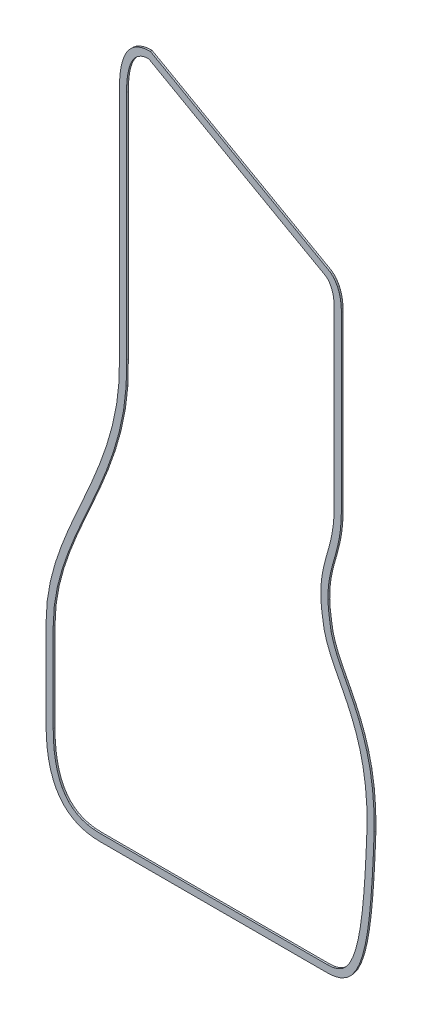
from build123d import *

# Parameters (mm, degrees)
EXTRUDE_1_DEPTH = 1.5


with BuildPart() as part:
    # 草图1 → 凸台-拉伸1 (new, symmetric)
    with BuildSketch(Plane.XY):
        Polygon((103, 235), (-24.833333333, 235), (-152.666666667, 235), (-280.5, 235), (-293.035714286, 235.637755102), (-304.642857143, 237.551020408), (-315.321428571, 240.739795918), (-325.071428571, 245.204081633), (-333.892857143, 250.943877551), (-341.785714286, 257.959183673), (-348.75, 266.25), (-354.785714286, 275.816326531), (-359.892857143, 286.658163265), (-364.071428571, 298.775510204), (-367.321428571, 312.168367347), (-369.642857143, 326.836734694), (-371.035714286, 342.780612245), (-371.5, 360), (-371.5, 410), (-371.5, 460), (-371.5, 510), (-369.607325073, 541.716472303), (-364.317784257, 572.711370262), (-356.214103499, 603.18148688), (-345.879008746, 633.32361516), (-333.895225948, 663.334548105), (-320.84548105, 693.411078717), (-307.3125, 723.75), (-293.879008746, 754.548104956), (-281.127733236, 786.002186589), (-269.641399417, 818.309037901), (-260.002733236, 851.665451895), (-252.794460641, 886.268221574), (-248.59930758, 922.314139942), (-248, 960), (-248, 1090), (-248, 1220), (-248, 1350), (-247.734693878, 1361.020408163), (-246.93877551, 1371.224489796), (-245.612244898, 1380.612244898), (-243.755102041, 1389.183673469), (-241.367346939, 1396.93877551), (-238.448979592, 1403.87755102), (-235, 1410), (-231.020408163, 1415.306122449), (-226.510204082, 1419.795918367), (-221.469387755, 1423.469387755), (-215.897959184, 1426.326530612), (-209.795918367, 1428.367346939), (-203.163265306, 1429.591836735), (-196, 1430), (-95.25, 1373.333333333), (5.5, 1316.666666667), (106.25, 1260), (108.93622449, 1257.887755102), (111.423469388, 1255.551020408), (113.711734694, 1252.989795918), (115.801020408, 1250.204081633), (117.691326531, 1247.193877551), (119.382653061, 1243.959183673), (120.875, 1240.5), (122.168367347, 1236.816326531), (123.262755102, 1232.908163265), (124.158163265, 1228.775510204), (124.854591837, 1224.418367347), (125.352040816, 1219.836734694), (125.650510204, 1215.030612245), (125.75, 1210), (125.75, 1113.333333333), (125.75, 1016.666666667), (125.75, 920), (125.280976676, 904.7303207), (123.987609329, 890.903790087), (122.040451895, 878.279883382), (119.610058309, 866.618075802), (116.866982507, 855.677842566), (113.981778426, 845.218658892), (111.125, 835), (108.467201166, 824.781341108), (106.17893586, 814.322157434), (104.430758017, 803.381924198), (103.393221574, 791.720116618), (103.236880466, 779.096209913), (104.13228863, 765.2696793), (106.25, 750), (108.586825802, 735.40451895), (112.60787172, 721.39941691), (118.007561953, 707.656705539), (124.4803207, 693.848396501), (131.720572157, 679.646501458), (139.422740525, 664.72303207), (147.28125, 648.75), (154.990524781, 631.39941691), (162.244989067, 612.343294461), (168.739067055, 591.253644315), (174.167182945, 567.802478134), (178.223760933, 541.66180758), (180.603225219, 512.503644315), (181, 480), (179.493440233, 443.170553936), (177.702623907, 409.752186589), (175.542274052, 379.635568513), (172.927113703, 352.711370262), (169.771865889, 328.870262391), (165.991253644, 308.002915452), (161.5, 290), (156.212827988, 274.752186589), (150.044460641, 262.150145773), (142.909620991, 252.084548105), (134.72303207, 244.44606414), (125.39941691, 239.125364431), (114.853498542, 236.013119534), align=None)
        Polygon((102.488112638, 247), (-280.194946957, 247), (-291.750952244, 247.587912357), (-301.939381157, 249.267323716), (-311.086304794, 251.998727096), (-319.269802794, 255.74574999), (-326.593723128, 260.511169524), (-333.159888318, 266.347289199), (-339.036641603, 273.343424062), (-344.243793611, 281.596517903), (-348.760192346, 291.184277455), (-352.542987561, 302.153921701), (-355.545052513, 314.525068478), (-357.724860294, 328.298579184), (-359.049809484, 343.465122112), (-359.5, 360.161748385), (-359.5, 509.642269246), (-357.667784005, 540.345601874), (-352.58062518, 570.154610665), (-344.725809735, 599.6889852), (-334.624273039, 629.149945379), (-322.816419258, 658.720300079), (-309.861390546, 688.578532611), (-296.353342604, 718.861557594), (-296.313283758, 718.952371204), (-282.879792504, 749.750476161), (-282.758090847, 750.039758799), (-270.006815337, 781.493840432), (-269.821096566, 781.98224042), (-258.334762746, 814.289091732), (-258.113047539, 814.977806451), (-248.474381358, 848.334220445), (-248.254924969, 849.21820836), (-241.046652374, 883.82097804), (-240.874915061, 884.880982175), (-236.679761999, 920.926900543), (-236.600824671, 922.123331459), (-236.001517091, 959.809191518), (-236, 960), (-236, 1349.855576478), (-235.745936561, 1360.408980867), (-235.004299927, 1369.917142837), (-233.791586112, 1378.49942522), (-232.135684832, 1386.142046515), (-230.074372439, 1392.836907278), (-227.655075816, 1398.589081066), (-224.929608639, 1403.427188481), (-221.940301554, 1407.412931261), (-218.697643362, 1410.640916791), (-215.159524231, 1413.219303203), (-211.230394325, 1415.234241616), (-206.78880716, 1416.719722273), (-201.726993031, 1417.654211036), (-198.822604235, 1417.819703275), (-101.132724138, 1362.874195859), (99.560345749, 1249.994718999), (101.10414032, 1248.780795063), (102.824421948, 1247.164612528), (104.420336245, 1245.378327184), (105.902872014, 1243.401612825), (107.276860816, 1241.213614463), (108.541403636, 1238.795152478), (109.691077442, 1236.130267554), (110.717477853, 1233.206949618), (111.610704573, 1230.017151632), (112.36055055, 1226.556324049), (112.957315286, 1222.822719029), (113.39227206, 1218.816655621), (113.657869227, 1214.539860213), (113.75, 1209.881350343), (113.75, 920.184252494), (113.298162249, 905.474072421), (112.073176816, 892.378567391), (110.228664628, 880.420135389), (107.911684915, 869.302523931), (105.261563225, 858.733020392), (102.419339497, 848.429645251), (99.568127134, 838.230896091), (99.511392219, 838.020614891), (96.853593386, 827.801955999), (96.744475573, 827.346044731), (94.456210267, 816.886861058), (94.329266723, 816.215657196), (92.581088881, 805.27542396), (92.477970552, 804.445348758), (91.440434108, 792.783541178), (91.394141727, 791.868719541), (91.23780062, 779.244812836), (91.261964854, 778.32071261), (92.157373017, 764.494181998), (92.246055168, 763.62120907), (94.363766539, 748.35152977), (94.400908642, 748.102887988), (96.737734444, 733.507406939), (97.052809357, 732.092953664), (101.073855275, 718.087851623), (101.439066208, 717.011047801), (106.838756441, 703.268336431), (107.142089161, 702.563425554), (113.614847908, 688.755116517), (113.789468159, 688.398105505), (121.029719617, 674.196210461), (121.057046388, 674.142937325), (128.706276206, 659.322039938), (136.410272188, 643.663068567), (143.891791488, 626.825074601), (150.891275708, 608.438737149), (157.144605916, 588.13092031), (162.376775049, 565.526305684), (166.298929877, 540.251860693), (168.609190582, 511.941724152), (168.997004903, 480.172117453), (167.506570621, 443.736875916), (165.725619763, 410.502607755), (163.583854895, 380.645075926), (161.003483151, 354.079041305), (157.913113026, 330.728150386), (154.253299546, 310.527560462), (149.986618519, 293.42483061), (145.114040864, 279.372676688), (139.693108872, 268.297654338), (133.827790213, 260.02305523), (127.559816514, 254.174732191), (120.664075373, 250.23954533), (112.621644342, 247.866113821), align=None, mode=Mode.SUBTRACT)
    extrude(amount=EXTRUDE_1_DEPTH, both=True)


solid = part.part
